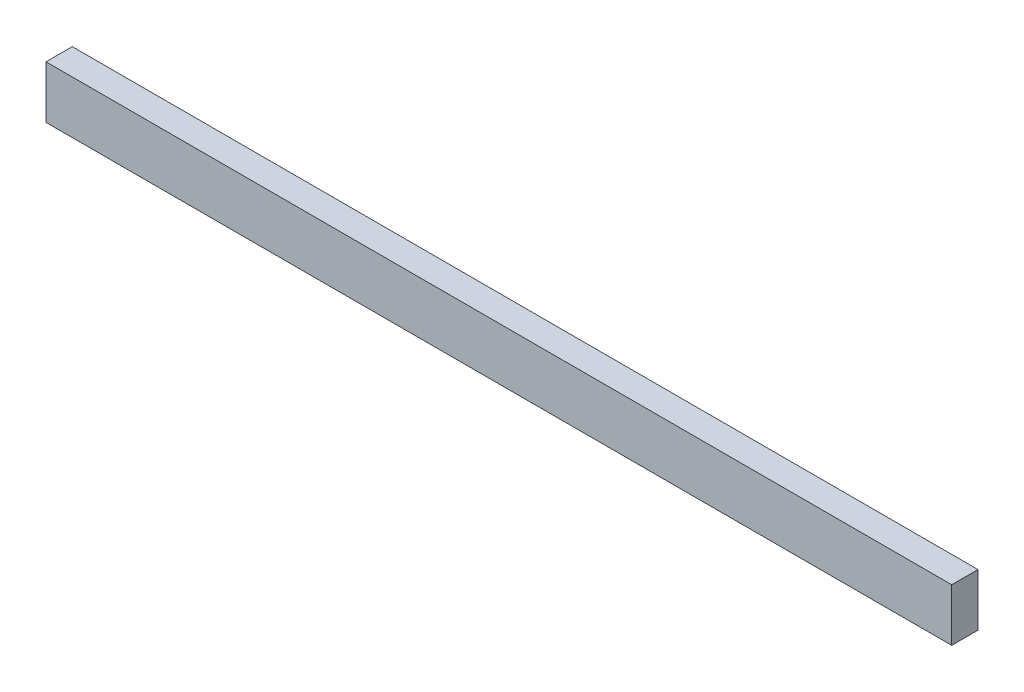
SolidWorks part; units mm, degrees
material "普通碳钢"
ref_plane "Front Plane" through (0, 0, 0) normal (0, 0, 1) x (1, 0, 0)
ref_plane "Top Plane" through (0, 0, 0) normal (0, 1, 0) x (1, 0, 0)
ref_plane "Right Plane" through (0, 0, 0) normal (1, 0, 0) x (0, 0, -1)
sketch "Sketch1" plane through (0, 0, 0) normal (0, 0, 1) x (1, 0, 0)
  line L1 (-172.5, 10) -> (172.5, 10)
  line L2 (-172.5, 10) -> (-172.5, -10)
  line L3 (-172.5, -10) -> (172.5, -10)
  line L4 (172.5, 10) -> (172.5, -10)
  line L5 (-172.5, 10) -> (172.5, -10) construction
  line L6 (-172.5, -10) -> (172.5, 10) construction
  point P0 (0, 0)
  dimension "D1" = 20
  dimension "D2" = 345
extrude "Boss-Extrude1" add sketch "Sketch1" along normal blind 10
